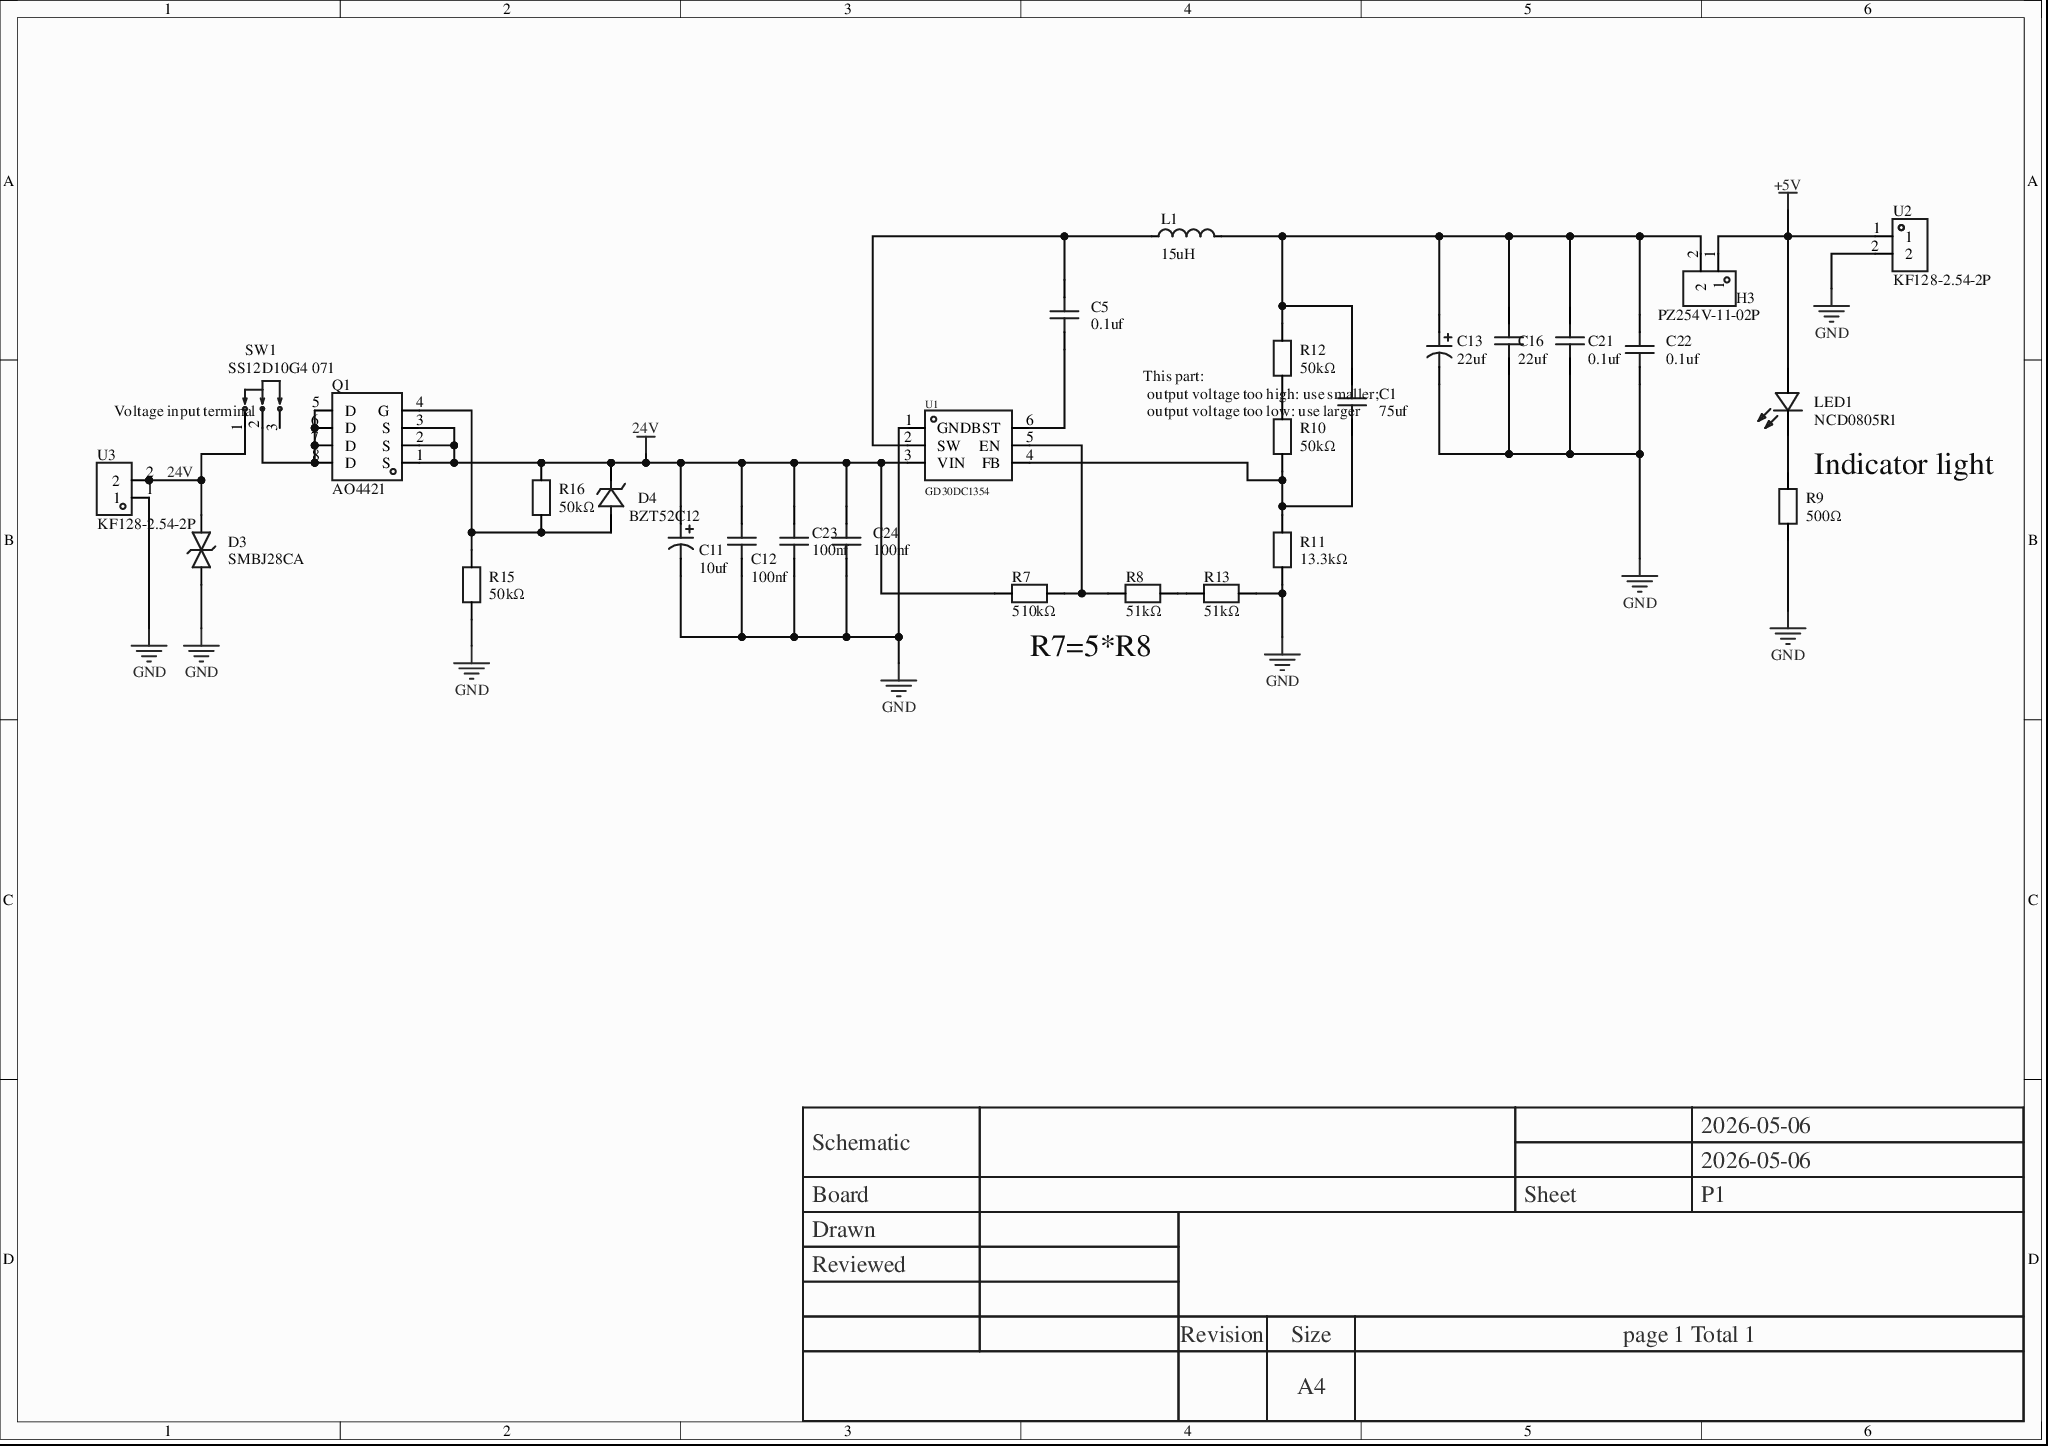
[diagram p0: MISC52037-3.schdoc]
# Altium project MISC52037.PrjPcb
1 sheet, 29 parts. Net scope: global (net labels, ports and power ports of the same name join across sheets).
Board file: MISC52037.pcbdoc

## Sheet MISC52037-3.schdoc
size 297 x 209 mm; Version: V1.0; @Project Name: MISC52037; @Update Date: 2026-05-18; @Create Date: 2026-05-18; @Board Name: MISC52037; @Create Time: 19:40:05; @Page Count: 1; @Page No: 1; @Schematic Name: MISC52037; @Update Time: 19:40:05; Size: A4

### Parts
C1  75uf  [C0603]
C5  0.1uf  [C0603]
C11  10uf  [CAP-SMD_BD6.3-L6.6-W6.6-FD]
C12  100nf  [CAP-TH_L5.0-W2.5-P5.00-D1.0]
C13  22uf  [CAP-SMD_BD6.3-L6.6-W6.6-FD]
C16  22uf  [CAP-TH_L5.0-W2.5-P5.00-D1.0]
C21  0.1uf  [C0603]
C22  0.1uf  [C0603]
C23  100nf  [C0603]
C24  100nf  [C0603]
D3  SMBJ28CA  [SMB_L4.6-W3.6-LS5.4-BI]
D4  BZT52C12  [SOD-123_L2.7-W1.6-LS3.7-RD]
H3  PZ254V-11-02P  [HDR-TH_2P-P2.54-V-M]
L1  15uH  [IND-SMD_L5.7-W5.2_GSM0530]
LED1  NCD0805R1  [LED0805-RD]
Q1  AO4421  [SOIC-8_L4.9-W3.9-P1.27-LS6.0-BL]
R7  510kΩ  [R0603]
R8  51kΩ  [R0603]
R9  500Ω  [R0603]
R10  50kΩ  [R0603]
R11  13.3kΩ  [R0603]
R12  50kΩ  [R0603]
R13  51kΩ  [R0603]
R15  50kΩ  [R0603]
R16  50kΩ  [R0603]
SW1  SS12D10G4 071  [SW-TH_SHOU-HAN_SS12D10G4]
U1  GD30DC1354  [SOT-23-6_L2.9-W1.7-P0.95-LS2.8-BL]
U2  KF128-2.54-2P  [CONN-TH_P2.54_KF128-2.54-2P]
U3  KF128-2.54-2P  [CONN-TH_P2.54_KF128-2.54-2P]

### Nets
24V: C11.1 C12.2 C23.1 C24.1 D3.2 D4.1(K) Q1.1(S) Q1.2(S) Q1.3(S) R7.2 R16.2 SW1.1 U1.3(VIN) U3.2
+5V: H3.1 LED1.2(+) U2.1
GND: C11.2 C12.1 C13.2 C16.1 C21.2 C22.2 C23.2 C24.2 D3.1 R9.1 R11.1 R13.1 R15.1 U1.1(GND) U2.2 U3.1
NetC1_1: C1.1 R10.1 R11.2 U1.4(FB)
NetC1_2: C1.2 C13.1 C16.2 C21.1 C22.1 H3.2 L1.2 R12.2
NetC5_1: C5.1 L1.1 U1.2(SW)
NetC5_2: C5.2 U1.6(BST)
NetD4_2: D4.2(A) Q1.4(G) R15.2 R16.1
NetLED1_1: LED1.1(-) R9.2
NetQ1_5: Q1.5(D) Q1.6(D) Q1.7(D) Q1.8(D) SW1.2
NetR7_1: R7.1 R8.2 U1.5(EN)
NetR8_1: R8.1 R13.2
NetR10_2: R10.2 R12.1

Not connected (* = marked no-connect by the designer): SW1 3

### Notes on the sheet
- (near SW1) Voltage input terminal
- This part:
  output voltage too high: use smaller;
  output voltage too low: use larger
- Indicator light
- R7=5*R8
- 2026-05-06
- Schematic
- Board
- Sheet
- P1
- Drawn
- Reviewed
- Revision
- Size
- A4
- page 1 Total 1

### Library data of the parts
C1 = CGA0603X7R104K500JT: Capacitance:100nF;Tolerance:±10%;Rated voltage:50V;Temperature coefficient:X7R;; Manufacturer: HRE(芯声); 3D Model: ac125912035d415993ca9572d50418b10819f05c4eef4c71ace90d822a990e87; 3D Model Transform: 62.992,31.496,0,0,0,0,0,0,0; Tolerance: ±10%; Voltage Rating: 50V; Temperature Coefficient: X7R; AddInBom: yes; ModelName: C0603_L1.6-W0.8-H0.8; Device: CGA0603X7R104K500JT; Symbol: CGA0603X7R104K500JT; Value: 75uf; LCSC Part Name: 100nF ±10% 50V; Manufacturer Part: CGA0603X7R104K500JT; Supplier Footprint: 0603; JLCPCB Part Class: Extended Part; Datasheet: https://item.szlcsc.com/datasheet/CGA0603X7R104K500JT/7062573.html; Supplier: LCSC; FootprintName: C0603; ConvertToPcb: yes
C5 C21-C24 = CL10A226MQ8NRNC: Capacitance:22uF;Tolerance:±20%;Rated voltage:6.3V;Temperature coefficient:X5R;; Manufacturer: SAMSUNG(三星); 3D Model: ac125912035d415993ca9572d50418b10819f05c4eef4c71ace90d822a990e87; 3D Model Transform: 62.992,31.496,0,0,0,0,0,0,0; Tolerance: ±20%; Voltage Rating: 6.3V; Temperature Coefficient: X5R; AddInBom: yes; ModelName: C0603_L1.6-W0.8-H0.8; Device: CL10A226MQ8NRNC; Symbol: CL10A226MQ8NRNC; LCSC Part Name: 22uF ±20% 6.3V; Manufacturer Part: CL10A226MQ8NRNC; Supplier Footprint: 0603; JLCPCB Part Class: Basic Part; Datasheet: https://item.szlcsc.com/datasheet/CL10A226MQ8NRNC/60514.html; Supplier: LCSC; FootprintName: C0603; ConvertToPcb: yes
  C5 C21 C22: Value: 0.1uf
  C23 C24: Value: 100nf
C11 C13 = RVT220UF16V67RV0015: Capacitance:220uF;Tolerance:±20%;Rated voltage:16V;Ripple current:110mA@120Hz;Equivalent series resistance (ESR):-;; Manufacturer: KNSCHA(科尼盛); 3D Model: ec7f1c7bda5e4386b54ec5ff3d1d94ff0819f05c4eef4c71ace90d822a990e87; 3D Model Transform: 307.086,259.842,0,180,0,0,0,0,0; Tolerance: ±20%; Voltage Rating: 16V; Lifetime: 2000hrs@105℃; AddInBom: yes; Device: RVT220UF16V67RV0015; Symbol: RVT220UF16V67RV0015; LCSC Part Name: 220uF ±20% 16V; Manufacturer Part: RVT220UF16V67RV0015; Supplier Footprint: SMD,D6.3xL7.7mm; JLCPCB Part Class: Extended Part; Datasheet: https://item.szlcsc.com/datasheet/RVT220UF16V67RV0015/3103841.html; Supplier: LCSC; Ripple Current: 110mA@120Hz; Equivalent Series Resistance(ESR): -; Diameter: 6.3mm; Height - Seated (Max): 7.7mm; Operating Temperature: -55℃~+105℃; FootprintName: CAP-SMD_BD6.3-L6.6-W6.6-FD; ConvertToPcb: yes; ModelName: CAP-SMD_BD6.3-L6.6-W6.6-FD
  C11: Value: 10uf
  C13: Value: 22uf
C12 C16 = CC1H104MC1FD3F6C10MF: Capacitance:100nF;Tolerance:±20%;Rated voltage:50V;Temperature coefficient:Y5V;; Manufacturer: Dersonic(德尔创); 3D Model: 08e3d7481fc7486bb1b263873f51e1e10819f05c4eef4c71ace90d822a990e87; 3D Model Transform: 224.652,98.425,0,0,0,0,-0.005,0,-137.795; Tolerance: ±20%; Voltage Rating: 50V; Pin Spacing: 5.08mm; Temperature Coefficient: Y5V; Body Thickness: 2.2mm; AddInBom: yes; ModelName: CAP-TH_BD5.0-W2.5-P5.08; Device: CC1H104MC1FD3F6C10MF; Symbol: CC1H104MC1FD3F6C10MF; LCSC Part Name: 100nF ±20% 50V; Manufacturer Part: CC1H104MC1FD3F6C10MF; Supplier Footprint: 插件,P=5.08mm; JLCPCB Part Class: Extended Part; Datasheet: https://item.szlcsc.com/datasheet/CC1H104MC1FD3F6C10MF/248635.html; Supplier: LCSC; Diameter: 6mm; FootprintName: CAP-TH_L5.0-W2.5-P5.00-D1.0; ConvertToPcb: yes
  C12: Value: 100nf
  C16: Value: 22uf
D3 = SMBJ28CA_C19077583: 极性:双向;反向截止电压(Vrwm):28V;钳位电压:45.4V;峰值脉冲电流(Ipp):13.22A@10/1000us;峰值脉冲功率(Ppp):600W@10/1000us;击穿电压:34.4V;; Manufacturer: R+O(宏嘉诚); AddInBom: yes; Polarity: Bidirectional; Reverse Stand-Off Voltage (Vrwm): 28V; Clamping Voltage: 45.4V; Voltage - Breakdown: 34.4V; Reverse Leakage Current (Ir): 5uA; level of protection: IEC 61000-4-2; Type: TVS; ModelId: 56a671846d664f15ac0751d5510bb56a0819f05c4eef4c71ace90d822a990e87; ModelTransform: 212.598,142.5194,0,0,0,0,0,0,0; Device: SMBJ28CA_C19077583; Symbol: SMBJ28CA_C19077583; FootprintName: SMB_L4.6-W3.6-LS5.4-BI; LCSC Part Name: 双向TVS 28V截止 峰值浪涌电流：13.22A@10/1000us; SupplierPart: C19077583; ManufacturerPart: SMBJ28CA; Supplier Footprint: DO-214AA(SMB); JLCPCB Part Class: Extended Part; Datasheet: https://item.szlcsc.com/datasheet/SMBJ28CA/20275668.html; Supplier: LCSC; ConvertToPcb: yes; Peak Pulse Current (Ipp): 13.22A@10/1000us; Peak Pulse Power Dissipation (Ppp): 600W@10/1000us; Operating Temperature: -55℃~+150℃; ModelName: SMB_L4.6-W3.6-LS5.4-BI
D4 = BZT52C12_C19077410: Diode configuration:Discrete;Zener voltage (nominal):12V;Zener voltage (range):11.4V~12.6V;Power dissipation (Pd):350mW;; Manufacturer: R+O(宏嘉诚); AddInBom: yes; Zener Voltage(Nom): 12V; Reverse Leakage Current (Ir): 100nA@8.0V; Pd - Power Dissipation: 350mW; Impedance(Zzt): 25Ω; Impedance(Zzk): 150Ω; Operating Junction Temperature Range: -55℃~+150℃; ModelId: ad7e39f9e5534b3c96ffdc5532ebb4930819f05c4eef4c71ace90d822a990e87; ModelName: SOD-123_L2.7-W1.6-H1.4-LS3.7; ModelTransform: 146.026,62.992,0,180,0,0,0.0005,0,0; Device: BZT52C12_C19077410; Symbol: BZT52C12_C19077410; FootprintName: SOD-123_L2.7-W1.6-LS3.7-RD; LCSC Part Name: 表面贴装齐纳二极管; SupplierPart: C19077410; ManufacturerPart: BZT52C12; Supplier Footprint: SOD-123; JLCPCB Part Class: Extended Part; Datasheet: https://item.szlcsc.com/datasheet/BZT52C12/20275495.html; Supplier: LCSC; ConvertToPcb: yes; Diode Configuration: Discrete; Zener Voltage(Range): 11.4V~12.6V
H3 = PZ254V-11-02P: 插针结构:1x2P;间距:2.54mm;行距:-;圆针/方针:方针;安装方式:直插;排数:单排;总PIN位数:2P;额定电流:3A;额定电压:250V;配合针长度:6mm;塑高:2.5mm;端接针长度:3mm;触头材质:黄铜;触头镀层:-;工作温度:-40℃~+105℃;颜色:黑色;; Manufacturer: XFCN(兴飞); 3D Model: e35305ec3aa84b66b849f914b715e73f0819f05c4eef4c71ace90d822a990e87; 3D Model Transform: 200,100,0,0,0,0,0,0,-118.11; Pin Structure: 1x2P; Pitch: 2.54mm; Circluar Pins/Square Pins: Square pin; Current Rating: 3A; Voltage Rating (Max): 250V; AddInBom: yes; ModelName: HDR2.54-M-LI-1X2P; Device: PZ254V-11-02P; Symbol: PZ254V-11-02P; LCSC Part Name: 1x2P 间距:2.54mm 方针 直插; Supplier Part: C492401; Manufacturer Part: PZ254V-11-02P; Supplier Footprint: 插件,P=2.54mm; JLCPCB Part Class: Extended Part; Datasheet: https://item.szlcsc.com/datasheet/PZ254V-11-02P/502957.html; Supplier: LCSC; Row Spacing: -; Mounting Type: Through-hole; Number of Rows: Single row; Number of Pins: 2P; Length of Mating Pin: 6mm; Insulation Height: 2.5mm; Length of End Connection Pin: 3mm; Contact Material: Brass; Contact Plating: -; Operating Temperature: -40℃~+105℃; Color: Black; FootprintName: HDR-TH_2P-P2.54-V-M; ConvertToPcb: yes
L1 = SRG0530-150-M: Inductance:15uH;Tolerance:±20%;Rated current:2.5A;Saturation current (Isat):3A;Type:Molded inductor;; Manufacturer: JIERR(捷而瑞); Tolerance: ±20%; Current Rating: 2.5A; Current - Saturation(Isat): 3A; DC Resistance(DCR): 218mΩ; AddInBom: yes; Device: SRG0530-150-M; Symbol: SRG0530-150-M; LCSC Part Name: 15μH ±20% 3A; Supplier Part: C53462979; Manufacturer Part: SRG0530-150-M; Supplier Footprint: SMD,5.7x5.2mm; JLCPCB Part Class: Extended Part; Datasheet: https://item.szlcsc.com/datasheet/SRG0530-150-M/56628174.html; Supplier: LCSC; Value: 15uH; Type: Molded inductor; FootprintName: IND-SMD_L5.7-W5.2_GSM0530; ConvertToPcb: yes
LED1 = NCD0805R1: 灯头类型:-;发光颜色:红色;正向压降(Vf):1.6V~2.6V;功率:65mW;正向电流:25mA;波长:615nm~630nm;二极管配置:独立二极管;透镜颜色:-;色温:-;发光强度:195mcd;发光角度:130°;载带方式:-;工作温度:-30℃~+85℃;; Manufacturer: 国星光电; Symbol: FC-2012HRK-620D; 3D Model: b1c5ed7a4f6e46d3bc6f6cc7c20f3fea0819f05c4eef4c71ace90d822a990e87; 3D Model Transform: 79.527,49.2125,0,0,0,0,0,0,0; Illumination Color: Red; Power(Watts): 65mW; Forward Current: 25mA; Peak Wavelength: 630nm; Diode Configuration: Discrete diode; Luminous Intensity: 195mcd; Viewing Angle: 130°; AddInBom: yes; Device: NCD0805R1; LCSC Part Name: 片式发光二极管; Supplier Part: C84256; Manufacturer Part: NCD0805R1; Supplier Footprint: 0805; JLCPCB Part Class: Basic Part; Datasheet: https://item.szlcsc.com/datasheet/NCD0805R1/85425.html; Supplier: LCSC; Lamp Holder Type: -; Voltage - Forward(Vf): 1.6V~2.6V; Wavelength - Dominant: 615nm~630nm; Lens Color: -; Color Temperature: -; Mounting Style: -; Operating Temperature: -30℃~+85℃; FootprintName: LED0805-RD; ConvertToPcb: yes; ModelName: LED0805-RD
Q1 = AO4421: 类型:P沟道;漏源电压(Vdss):60V;连续漏极电流(Id):6.2A;功率(Pd):3.1W;导通电阻(RDS(on)@Vgs,Id):40mΩ@10V,6.2A;阈值电压(Vgs(th)@Id):3V@250uA;; Manufacturer: AOS; AddInBom: yes; Type: P-channel; Drain Source Voltage (Vdss): 60V; Power Dissipation (Pd): 3.1W; Total Gate Charge (Qg@Vgs): 55nC@10V; Input Capacitance (Ciss@Vds): 2.9nF@30V; ModelId: e81d2f7d937b4a6ab1dca543ff5d56a40819f05c4eef4c71ace90d822a990e87; ModelName: SOIC-8_L4.9-W3.9-H1.7-LS6.0-P1.27; ModelTransform: 192.913,236.22,0,0,0,0,0,0,0; Device: AO4421; Symbol: AO4421; FootprintName: SOIC-8_L4.9-W3.9-P1.27-LS6.0-BL; LCSC Part Name: P沟道 耐压:60V 电流:6.2A; SupplierPart: C33484; ManufacturerPart: AO4421; Supplier Footprint: SOIC-8; JLCPCB Part Class: Extended Part; Datasheet: https://atta.szlcsc.com/upload/public/pdf/source/20180704/C33484_0DEC87524387A472D57ED5D386F8FCE9.pdf; Supplier: LCSC; ConvertToPcb: yes; Continuous Drain Current (Id): 6.2A; Drain Source On Resistance (RDS(on)@Vgs,Id): 40mΩ@10V,6.2A; Gate Threshold Voltage (Vgs(th)@Id): 3V@250uA; Operating Temperature: -55℃~+150℃@(Tj)
R7-R13 R15 R16 = FRC0603F1002TS: Resistor type:Thick film resistor;Resistance:10kΩ;Tolerance:±1%;Power:100mW;Working voltage:75V;Temperature coefficient:±100ppm/℃;; Manufacturer: FOJAN(富捷); AddInBom: yes; Tolerance: ±1%; Power(Watts): 100mW; Voltage-Supply(Max): 75V; ModelId: fc143cca1e79419f9cd78b61e9279f080819f05c4eef4c71ace90d822a990e87; ModelTransform: 31.8897,63.7794,0,90,0,0,0,0,0; Device: FRC0603F1002TS; Symbol: FRC0603F1002TS; FootprintName: R0603; LCSC Part Name: 10kΩ ±1% 100mW 厚膜电阻; ManufacturerPart: FRC0603F1002TS; Supplier Footprint: 0603; JLCPCB Part Class: Extended Part; Supplier: LCSC; ConvertToPcb: yes; Type: Thick film resistor; Temperature Coefficient: ±100ppm/℃; Operating Temperature: -55℃~+155℃; ModelName: R0603
  R7: Value: 510kΩ
  R8 R13: Value: 51kΩ
  R9: Value: 500Ω
  R10 R12 R15 R16: Value: 50kΩ
  R11: Value: 13.3kΩ
SW1 = SS12D10G4 071: Circuit structure:SPDT;Mounting:Through-hole;Switch color:-;Rated current:2A;Rated voltage:125V;Operating life:3 thousand cycles;; Manufacturer: SHOU HAN(首韩); 3D Model: cfce8581009a45839cc96a3fa85751f80819f05c4eef4c71ace90d822a990e87; 3D Model Transform: 499.999,263.779,0,0,0,0,-0.589,-0.591,-196.85; Circuit: SPDT; Switch Height: 6.4mm; Current Rating: 2A; Voltage Rating: 125V; AddInBom: yes; Device: SS12D10G4 071; Symbol: SS12D10G4 071; LCSC Part Name: SS12D10G4-7.0脚长; Supplier Part: C2887259; Manufacturer Part: SS12D10G4 071; Supplier Footprint: 插件,12.7x6.7mm; JLCPCB Part Class: Extended Part; Datasheet: https://item.szlcsc.com/datasheet/SS12D10G4%2520071/3103827.html; Supplier: LCSC; Actuator Style: -; Termination Style: PC pin; Length: 12.7mm; Width: 6.7mm; Mounting Type: Through-hole; Actuator Color: -; Life: 3 thousand cycles; Operating Temperature: -; FootprintName: SW-TH_SHOU-HAN_SS12D10G4; ConvertToPcb: yes; ModelName: SW-TH_SHOU-HAN_SS12D10G4
U1 = GD30DC1354: Manufacturer: null; ModelId: f198fe6923cc4b1fabccb73198a22cca0819f05c4eef4c71ace90d822a990e87; Device: GD30DC1354; Symbol: GD30DC1354; Supplier: LCSC; Supplier Part: C9900263753; Manufacturer Part: GD30DC1354; supplierPart: C9900263753; manufacturer: null; FootprintName: SOT-23-6_L2.9-W1.7-P0.95-LS2.8-BL; ModelName: SOT-23-6_L2.9-W1.7-P0.95-LS2.8-BL
U2 U3 = KF128-2.54-2P: Structure:1x2P;Pitch:2.54mm;Color:Green;Mounting:Through-hole;Rated current:8A;Rated voltage:130V;Rows:1;Wire gauge - AWG:18~26;Wire gauge - mm2:1;Pins per row:2;Operating temperature range:-40℃~+105℃;; Manufacturer: KEFA(科发); 3D Model: 38629642489141faa979009e13fb8a570819f05c4eef4c71ace90d822a990e87; 3D Model Transform: 200,248.031,0,0,0,0,0,-5.906,-137.795; Structure: 1x2P; Pitch: 2.54mm; Current Rating (Max): 8A; Voltage Rating (Max): 130V; Wire Gauge - AWG: 18~26; Wire Gauge - mm2: 1; Number of PINs Per Row: 2; AddInBom: yes; Device: KF128-2.54-2P; Symbol: KF128-2.54-2P; LCSC Part Name: 2.54mm 1x2P 排数:1 每排P数:2 直插; Supplier Part: C474920; Manufacturer Part: KF128-2.54-2P; Supplier Footprint: 插件,P=2.54mm; JLCPCB Part Class: Extended Part; Datasheet: https://atta.szlcsc.com/upload/public/pdf/source/20230317/0E5ECA9DB49110BC3219D12632CEA6EE.pdf; Supplier: LCSC; Color: Green; Mounting Style: Through-hole; Number of Pins: 2P; Number of Rows: 1; Operating Temperature Range: -40℃~+105℃; FootprintName: CONN-TH_P2.54_KF128-2.54-2P; ConvertToPcb: yes; ModelName: CONN-TH_P2.54_KF128-2.54-2P